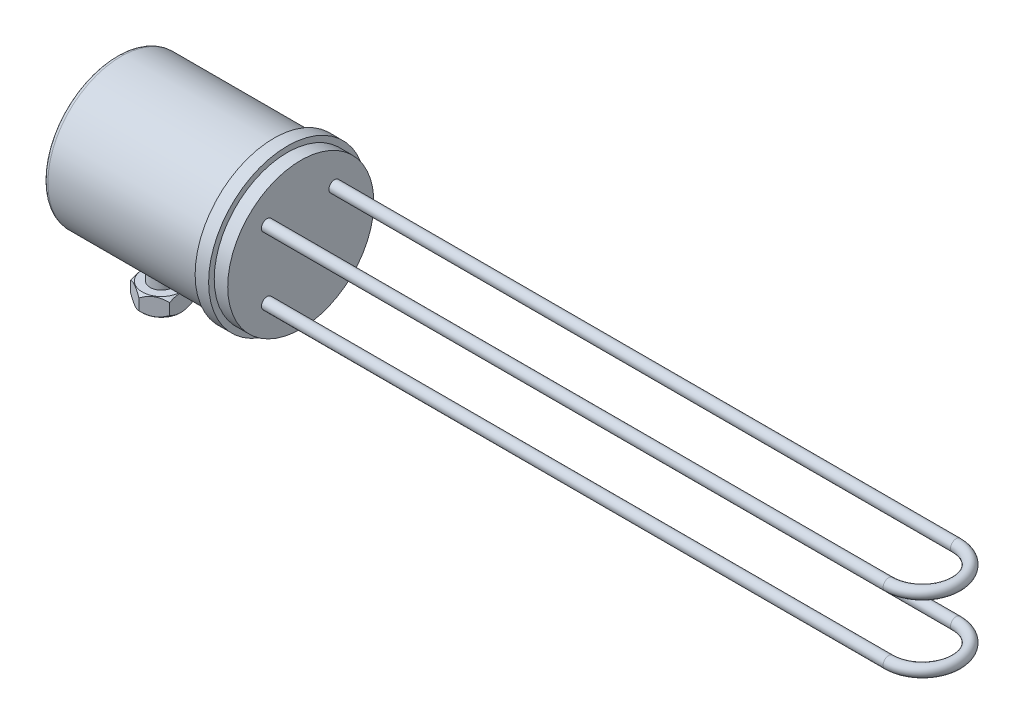
SolidWorks part; units mm, degrees
ref_plane "Front Plane" through (0, 0, 0) normal (0, 0, 1) x (1, 0, 0)
ref_plane "Top Plane" through (0, 0, 0) normal (0, 1, 0) x (1, 0, 0)
ref_plane "Right Plane" through (0, 0, 0) normal (1, 0, 0) x (0, 0, -1)
sketch "Sketch1" plane through (0, 0, 0) normal (1, 0, 0) x (0, 0, -1)
  circle A0 centre (0, 0) radius 2.5
  dimension "D1" = 5
sketch "Sketch2" plane through (0, 0, 0) normal (0, 1, 0) x (1, 0, 0)
  line L0 (0, 0) -> (282.5, 0)
  line L1 (297.5, 15) -> (300, 15) construction
  line L2 (282.5, 30) -> (0, 30)
  arc A0 (282.5, 0) -> (282.5, 30) centre (282.5, 15) ccw
  dimension "D1" = 2.5
  dimension "D2" = 30
  dimension "A" = 300
sweep "Sweep1" add profiles "Sketch1" path "Sketch2"
ref_plane "Plane1" through (0, -15, 0) normal (0, 1, 0) x (-1, 0, 0)
sketch "Sketch3" plane through (0, 0, 0) normal (-1, 0, 0) x (0, 0, 1)
  line L0 (-30, -30) -> (0, 0) construction
  line L1 (-30, 0) -> (0, 0) construction
  line L2 (-30, 0) -> (-30, -30) construction
  line L3 (-30, -30) -> (0, -30) construction
  line L4 (0, 0) -> (0, -30) construction
  circle A0 centre (-15, -15) radius 32.5
  dimension "D1" = 65
extrude "Boss-Extrude1" add sketch "Sketch3" against normal blind 6
mirror "Mirror3" about plane through (0, -15, 0) normal (0, 1, 0) of "Sweep1"
sketch "Sketch4" plane through (0, -15, 0) normal (0, 1, 0) x (-1, 0, 0)
  line L0 (0, -15) -> (0, 42.5)
  line L1 (0, -47.5) -> (0, 17.5) construction
  line L2 (0, 42.5) -> (6, 42.5)
  line L3 (6, 42.5) -> (6, 17.5)
  line L4 (6, 17.5) -> (76, 17.5)
  line L5 (76, 17.5) -> (76, -5)
  line L6 (78, -15) -> (0, -15)
  line L7 (76, -5) -> (78, -5)
  line L8 (78, -5) -> (78, -15)
  arc A0 (-282.5, 2.5) -> (-282.5, -32.5) centre (-282.5, -15) ccw construction
  dimension "D1" = 6
  dimension "B" = 376
  dimension "D2" = 2
  dimension "D3" = 10
  dimension "D4" = 32.5
  dimension "D5" = 57.5
revolve "Revolve1" add sketch "Sketch4" angle 360 about L6
sketch "Sketch5" plane through (-6, 0, 0) normal (-1, 0, 0) x (0, 0, 1)
  circle A0 centre (-15, -15) radius 47 construction
  circle A1 centre (-15, 32) radius 4.5
  dimension "D1" = 94
  dimension "D2" = 9
extrude "Cut-Extrude1" cut sketch "Sketch5" against normal up to surface (6 mm away) up to face at (0, -15, 17.5)
pattern_circular "CirPattern1" count 6 over 360 about axis through (0, -15, -15) along (1, 0, 0) of "Cut-Extrude1"
sketch "Sketch6" plane through (0, -15, 0) normal (0, 1, 0) x (-1, 0, 0)
  line L0 (0, -15) -> (78, -15) construction
  line L1 (0, 42.5) -> (0, -72.5) construction
  line L2 (78, -25) -> (78, -5) construction
  line L3 (76, -47.5) -> (76, 17.5) construction
  circle A0 centre (56, -15) radius 5
  dimension "D1" = 20
  dimension "D2" = 10
extrude "Boss-Extrude2" add sketch "Sketch6" against normal blind 45
sketch "Sketch7" plane through (0, -60, 0) normal (0, -1, 0) x (1, 0, 0)
  circle A0 centre (-56, -15) radius 10
  dimension "D1" = 20
extrude "Boss-Extrude3" add sketch "Sketch7" along normal blind 8
chamfer "Chamfer1" distance 1.5 angle 45 2 edges at (-56, -60, -25) (-56, -68, -25)
sketch "Sketch8" plane through (0, -68, 0) normal (0, -1, 0) x (1, 0, 0)
  line L1 (-56, -5) -> (-64.6603, -10)
  line L2 (-64.6603, -10) -> (-64.6603, -20)
  line L3 (-64.6603, -20) -> (-56, -25)
  line L4 (-56, -25) -> (-47.3397, -20)
  line L5 (-47.3397, -20) -> (-47.3397, -10)
  line L6 (-47.3397, -10) -> (-56, -5)
  circle A0 centre (-56, -15) radius 8.6603 construction
  circle A1 centre (-56, -15) radius 10
  circle A2 centre (-56, -15) radius 10 construction
extrude "Cut-Extrude2" cut sketch "Sketch8" against normal blind 8 contours L2 A1 | L1 A1 | L6 A1 | L5 A1 | L4 A1 | L3 A1
fillet "Fillet1" radius 2 1 edges at (-76, -15, 17.5)
sketch "Sketch9" plane through (-6, 0, 0) normal (-1, 0, 0) x (0, 0, 1)
  circle A0 centre (-15, -15) radius 35
  circle A1 centre (-15, -15) radius 57.5 construction
  circle A2 centre (-15, -15) radius 57.5
  dimension "D1" = 70
extrude "Cut-Extrude3" cut sketch "Sketch9" against normal through all
